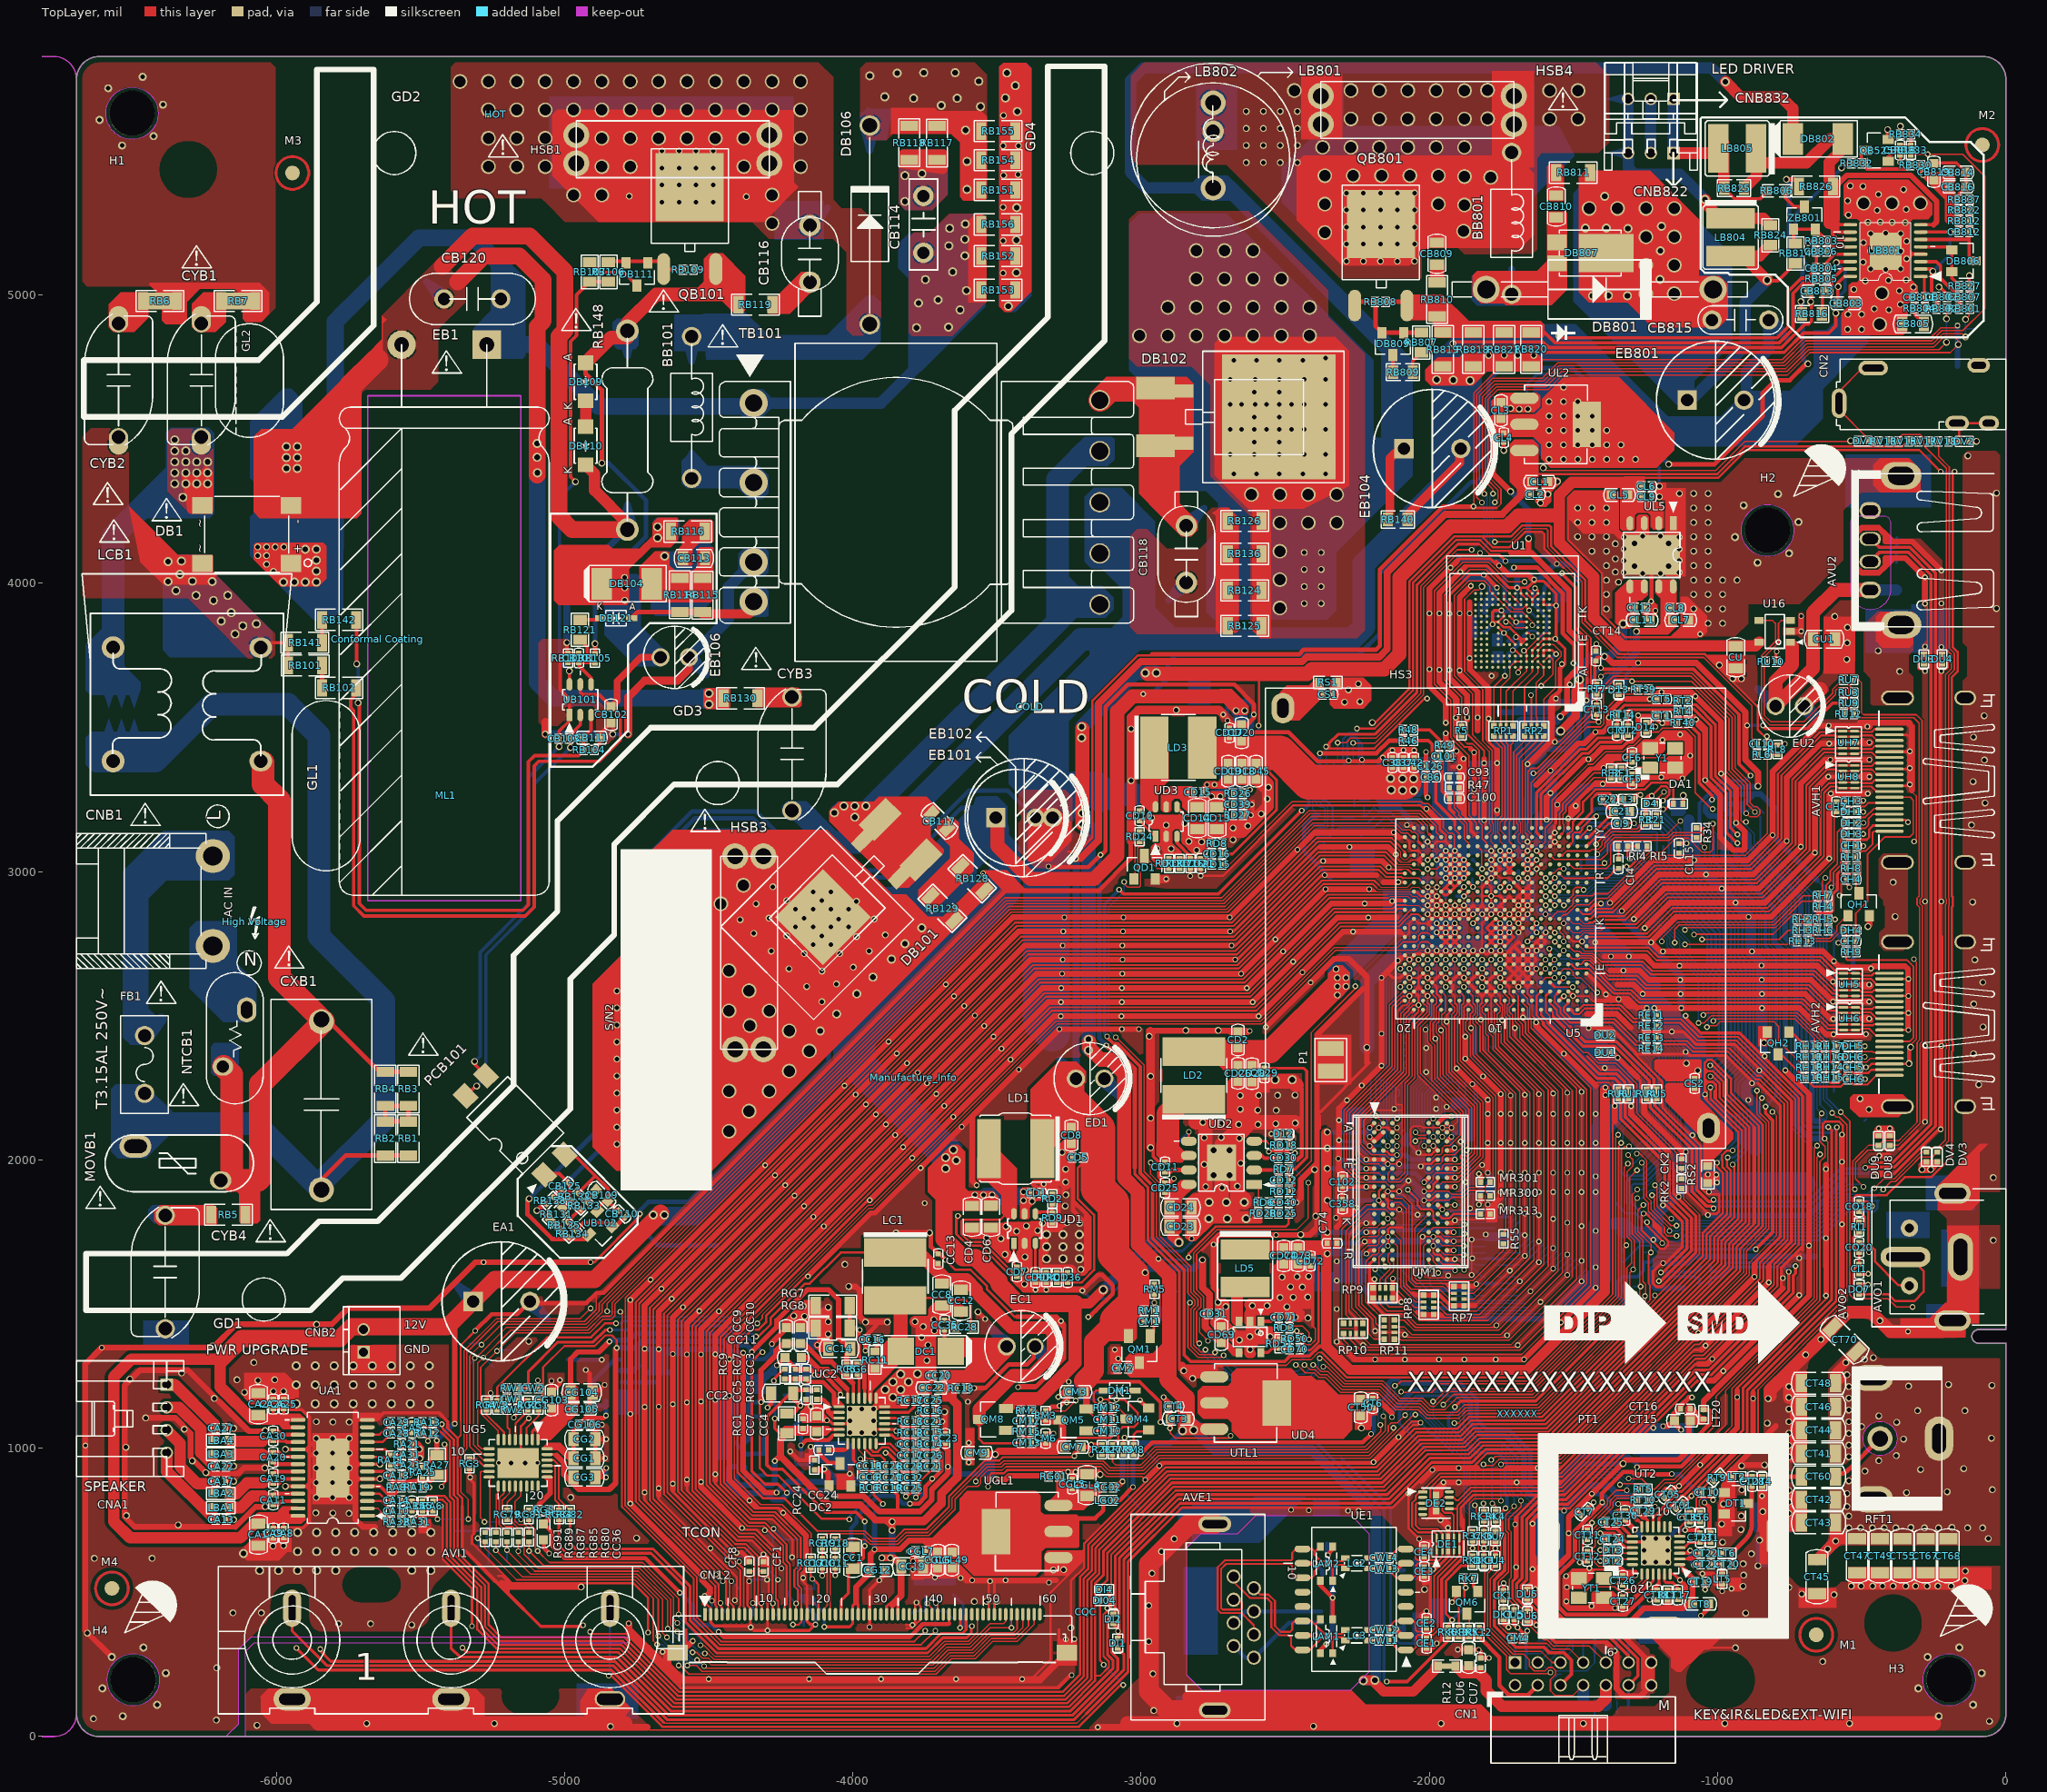
[diagram p0: TopLayer view]
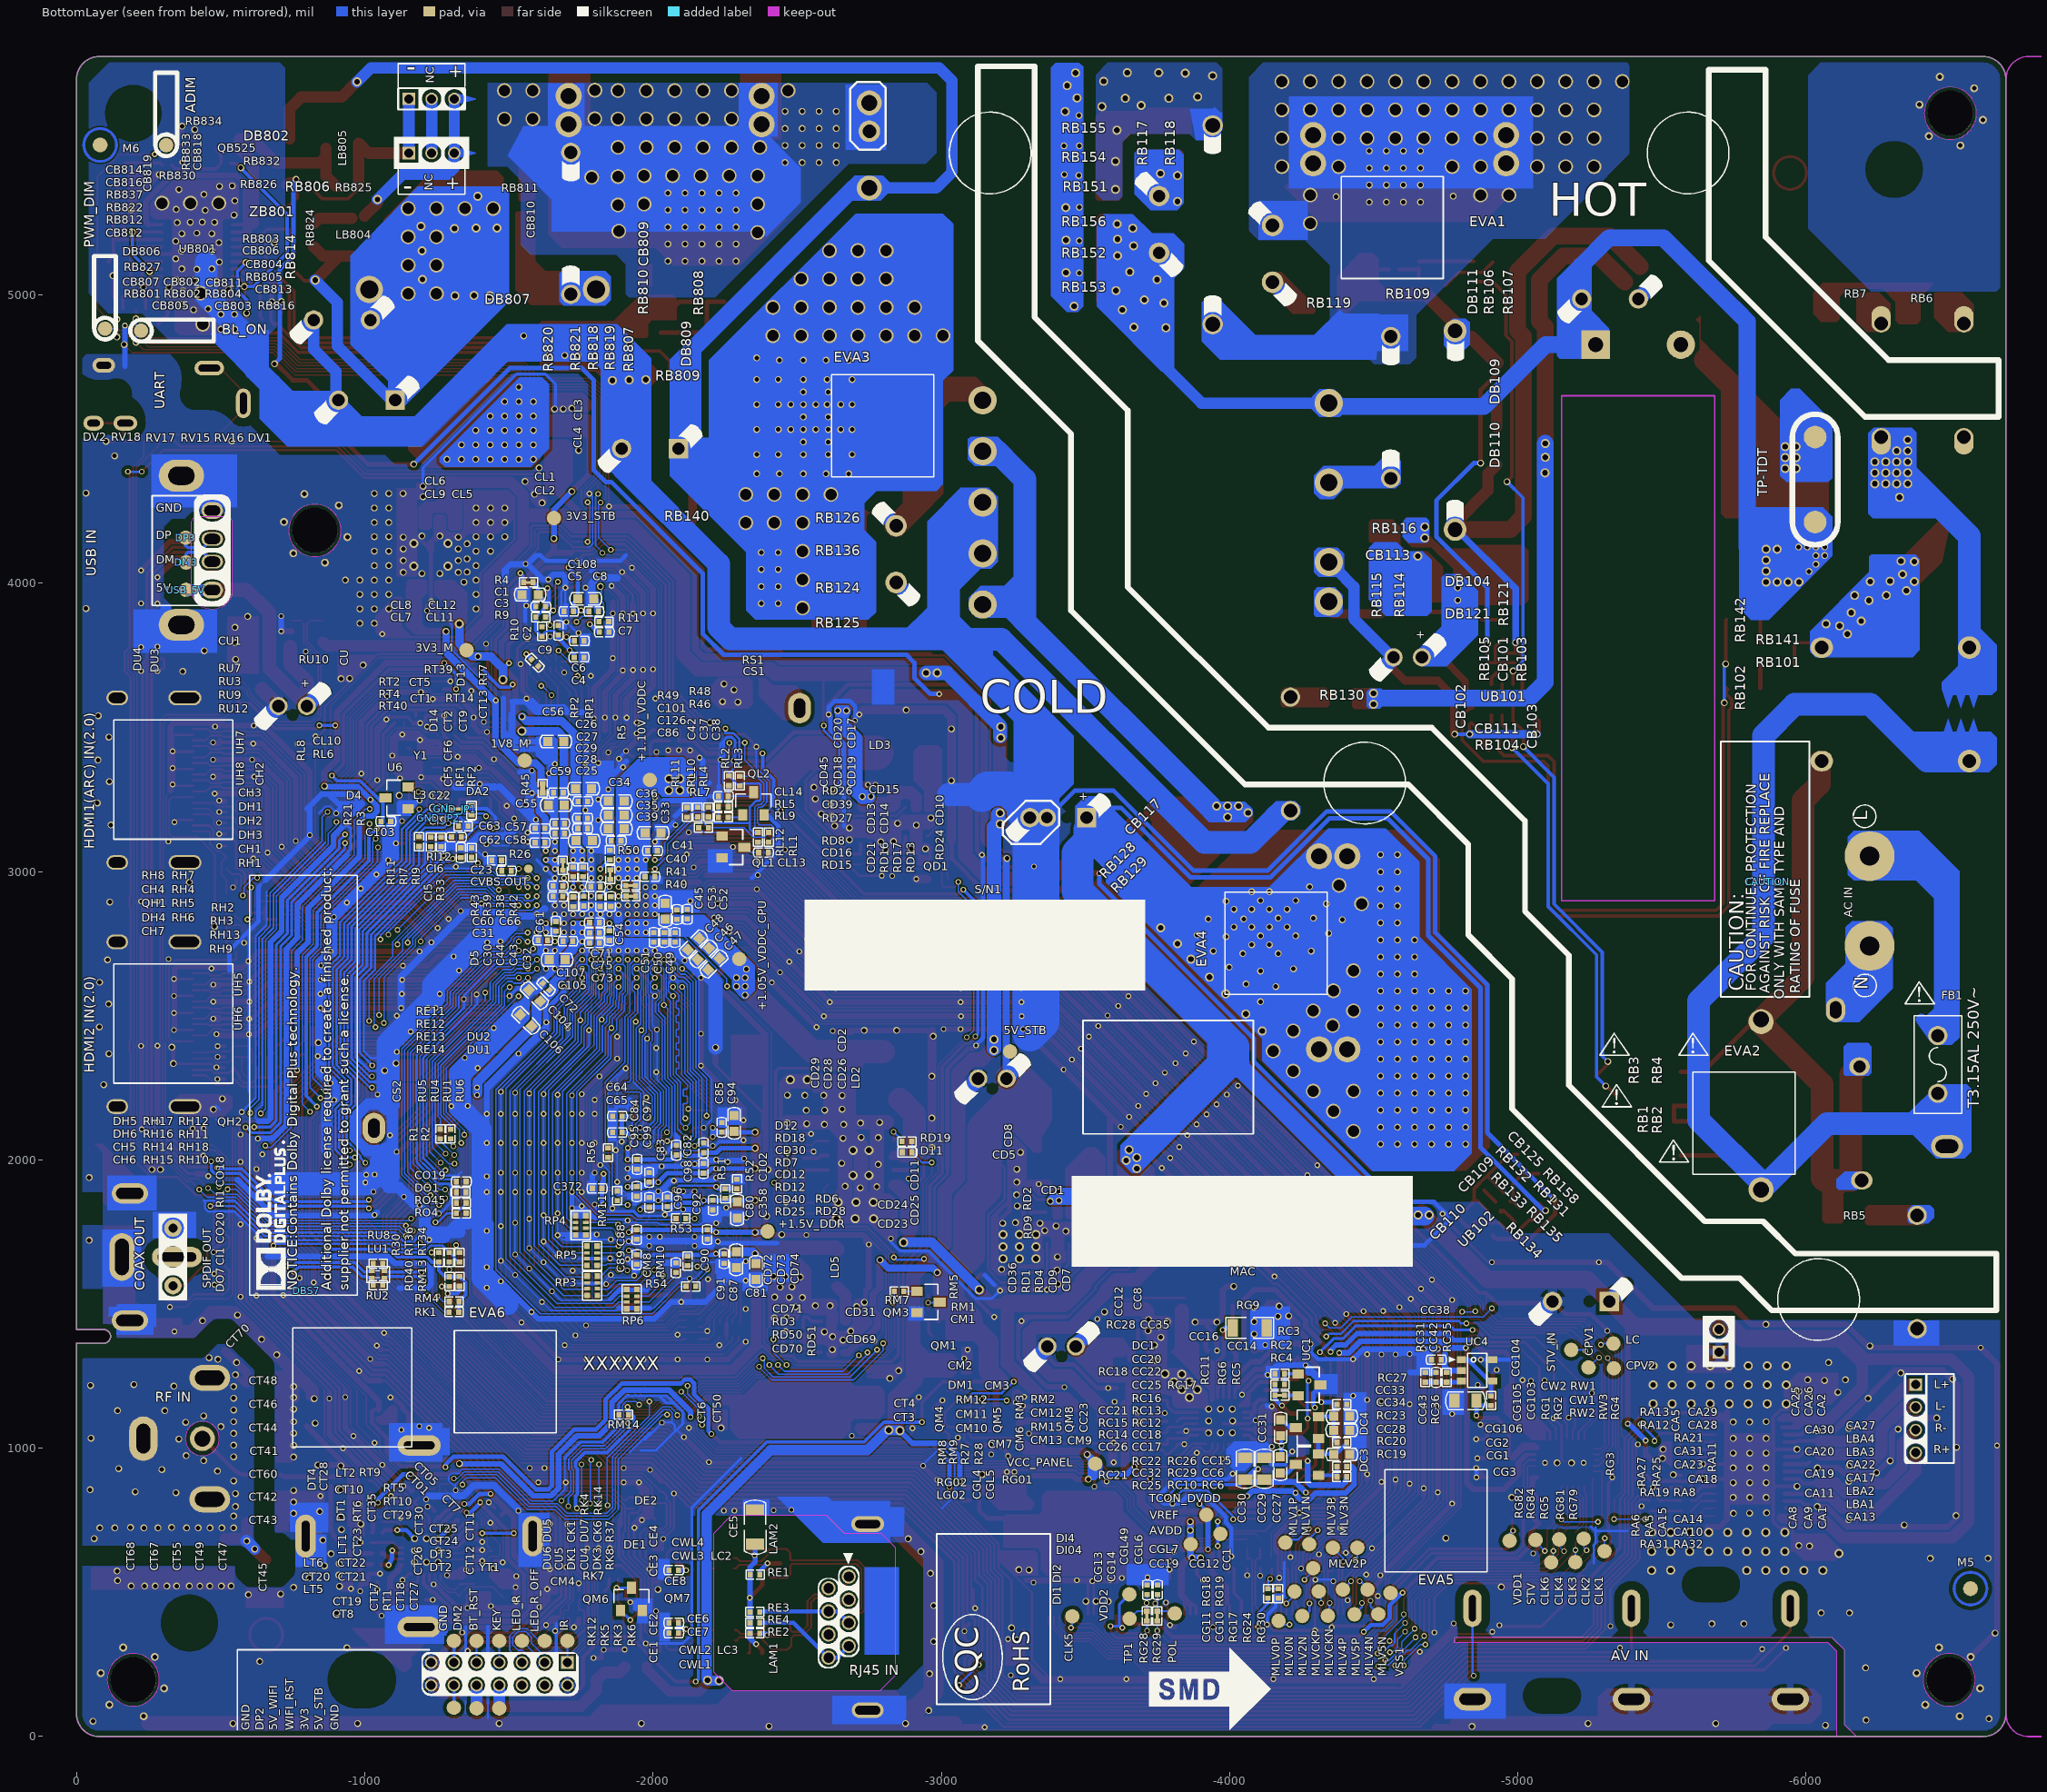
[diagram p1: BottomLayer view, seen from below]
# Altium PCB MISC84395.PcbDoc (part 1 of 26)
Units mil, origin at the board's own origin, x right, y up, seen from the top; angles counter-clockwise.
Board outline 6692.91 x 5826.77 mil, 2 copper layers (TopLayer, BottomLayer), stack 61.855 mil thick; 951 components, 565 nets, 4374 pads, 1804 vias.
Unrouted connection lines stored in the file: 1.

## Layer stack, top to bottom
TopLayer: signal copper 1.4
Dielectric: core 59.055, FR-4, Dk 4.8
BottomLayer: signal copper 1.4

## Board outline
-6692.91,78.74 -6692.91,5748.03 cw(c-6614.17,5748.03) -6614.17,5826.77 -78.74,5826.77 cw(c-78.74,5748.03) 0,5748.03 0,1411.42 -94.49,1411.42 ccw(c-94.49,1387.8) -118.11,1387.8 ccw(c-94.49,1387.8) -94.49,1364.17 0,1364.17 0,78.74 cw(c-78.74,78.74) -78.74,0 -6614.18,0 -6614.17,0 cw(c-6614.17,78.74)

## Design rules (kind name [scope] priority, off if disabled: settings)
Clearance ■KEEPOUT_18mil [(IsTrack Or IsArc) And (AsMM(Width) < 1) And IsKeepOut vs Not IsPad] p1: gap=18
Clearance ■HOT_7.2mm [InNetClass('HOT') vs InNetClass('All Nets') And (Not InNetClass('HOT'))] p2: gap=283.46
Clearance ■DFM_NPTH_10mil [(IsPadHoleValid And (PadIsPlated=false) Or IsPad And ((AsMM(PadXSize_AllLayers) < 1) or (AsMM(PadYSize_AllLayers) < 1 )) And IsKeepout) OR HasFootprintPad('ASSE*','0') vs Not IsPad] p3: gap=10
Clearance ■DFM_20mil [(IsTrack or IsArc or IsPad) And IsKeepOut vs IsTrack or IsArc or InPoly] p4: gap=20
Clearance ■C_RJ45_2mm [InNetClass('RJ45') vs Not InNetClass('RJ45') AND InNet('*')] p5: gap=78.74
Clearance ■PWR_A12_8mil [((InNetClass('PWR_A12_8mil') or InNet('*12V*') or InNet('*24V*') or InNet('*PVCC*') or InNet('*19V*') or InNet('*AMP*POWER*') or InNet('*AMP*VCC*') or InNet('*VGH*') or InNet('AVDD') or InNet('AVDD_SOURCE')) And Not InNetClass('A12_8mil_EXC')) and Not IsPad vs Not InPoly] p6: gap=8
Clearance ■PS_L2All_3.2mm [InNet('L-1') vs InNet('*')] p7: gap=125.98
Clearance ■PS_L2LN_1.5mm [InNet('L') Or InNet('L-2') Or InNet('L-3') Or InNet('L-4') Or InNet('L-5') Or InNet('L-6') vs InNet('L-N') And Not(InNet('L') Or InNet('L-2') Or InNet('L-3') Or InNet('L-4') Or InNet('L-5') Or InNet('L-6'))] p8: gap=59.06
Clearance ■PS_N2LN_1.5mm [InNet('N') OR InNet('N-1') OR InNet('N-2') OR InNet('N-3') OR InNet('N-4') OR InNet('N-5') OR InNet('N-6') vs InNet('L-N') And Not (InNet('N') OR InNet('N-1') OR InNet('N-2') OR InNet('N-3') OR InNet('N-4') OR InNet('N-5') OR InNet('N-6'))] p9: gap=59.06
Clearance ■PS_L2LN_3mm [InNet('L') Or InNet('L-2') Or InNet('L-3') Or InNet('L-4') Or InNet('L-5') Or InNet('L-6') vs InNet('*') And Not (InNet('L-N') Or InNet('L') Or InNet('L-2') Or InNet('L-3') Or InNet('L-4') Or InNet('L-5') Or InNet('L-6') Or OnLayer('KeepOutLayer'))] p10: gap=118.11
Clearance ■PS_N2LN_3mm [InNet('N') OR InNet('N-1') OR InNet('N-2') OR InNet('N-3') OR InNet('N-4') OR InNet('N-5') OR InNet('N-6') vs InNet('*') And Not (InNet('L-N') Or InNet('N') OR InNet('N-1') OR InNet('N-2') OR InNet('N-3') OR InNet('N-4') OR InNet('N-5') OR InNet('N-6') Or OnLayer('KeepOutLayer'))] p11: gap=118.11
Clearance ■SIP2GND_8mil [HasFootprint('SIP*') vs InPoly] p12: gap=8
Clearance ■C_BGA_0P65 [HasFootprint('BGA*0.65*') vs InPoly] p13: gap=5
Clearance ■C_BGA_0P8 [HasFootprint('BGA*0.8*') vs InPoly] p14: gap=5.5
Clearance ■Poly_4mil [InPolygonClass('Poly_4mil') vs Not InPoly] p15: gap=4
Clearance ■Poly_5mil [InPolygonClass('Poly_5mil') vs Not InPoly] p16: gap=5
Clearance ■Poly_6.2mil [InPolygonClass('Poly_6.2mil') vs Not InPoly] p17: gap=6.2
Clearance ■Poly_8mil [InPolygonClass('Poly_8mil') vs Not InPoly] p18: gap=8
Clearance ■C_RFGND_1.8mm [InNet('RFGND') vs Not (InNet('*RF*IN*') OR InNet('RF'))] p19: gap=70.87
Clearance ■ESD_10mil [HasFootprint('*IEC*') Or HasFootprint('*-F1*') Or HasFootprint('ANT-RF*')] p20: gap=10
Clearance ■ESD_20mil [HasFootprint('*SHIELD*')] p21: gap=20
Clearance ■GND_12mil [InNet('GND') vs InPoly] p22: gap=12
Clearance ■ESD_30mil [(HasFootprint('SCART*') OR HasFootprint('AV*') OR HasFootprint('DB15*') OR HasFootprint('PHONE*')) vs OnBottomLayer] p23: gap=30
Clearance ■ESD_NT_30mil [HasFootprint('SCART*') Or HasFootprint('PHONE-HD-12') Or HasFootprint('PHONE-HD-17') Or HasFootprint('PHONE-HD-10') Or HasFootprint('PHONE-HD-26') vs InNet('GND') And OnTopLayer] p24: gap=30
Clearance ■DFM_TH_5mil [HasFootprint('GND') or HasFootprint('TP*') or HasFootprint('MARK*') or HasFootprint('SPARK_GAP') or HasFootprint('USB-HD-3-2') or HasFootprint('PHONE-HS-20') and Not IsRegion vs OnBottomlayer And IsPad OR IsPadHoleValid] p25: gap=5
Clearance ■DFM_HS60_5mil [InPadClass('HS60') vs InPadClass('HS60') OR IsPadHoleValid and not InPadClass('VIA5')] p26: gap=5
Clearance ■DFM_BCR_4mm [IsPadHoleValid vs IsBoardCutoutRegion] p27: gap=157.48
Clearance ■DFM_TH_4mm [OnBottomlayer And IsSMTPin vs IsPadHoleValid and not InPadClass('VIA5')] p28: gap=157.48
Clearance ■DFM_HS60_4mm [InPadClass('HS60') vs IsPad and OnBottomlayer] p29: gap=157.48
Clearance ■VIA2VIA_6.2mil [(IsVia OR InPadClass('VIA5')) And Not (IsVia And (AsMM(HoleDiameter) = 0.1)) vs (IsVia OR InPadClass('VIA5')) And Not (IsVia And (AsMM(HoleDiameter) = 0.1))] p30: gap=6.2
Clearance ■VIA2VIA_10.2mil [(IsVia OR InPadClass('VIA5')) And Not (IsVia And (AsMM(HoleDiameter) = 0.1)) vs (IsVia OR InPadClass('VIA5')) And Not (IsVia And (AsMM(HoleDiameter) = 0.1))] p31: gap=10.2
Clearance ■VIA2PAD_BGA_5mil [HasFootprint('BGA*') and IsPad vs (IsVia OR InPadClass('VIA5')) And Not (IsVia And (AsMM(HoleDiameter) = 0.1))] p32: gap=4
Clearance ■VIA2PAD_6mil [IsVia And Not (IsVia And (AsMM(HoleDiameter) = 0.1)) vs ISPAD and Not HasFootprintPad('*','EPAD') and Not HasFootprintPad('*','257') and Not HasFootprintPad('TP','*') and Not HasFootprintPad('GND','JP*') and Not HasFootprintPad('LQFP216/0.4-2','217') and Not HasFootprintPad('QFP16*','17') and Not HasFootprintPad('QFN16*','17') and Not HasFootprintPad('QFN20*','21') and Not HasFootprintPad('QFN24*','25') and Not HasFootprintPad( 'QFN24*','29') and Not HasFootprintPad('QFN28*','29') and Not HasFootprintPad('QFN32*','33') and Not HasFootprintPad('QFN36*','37') and Not HasFootprintPad('QFN36*','0') and Not HasFootprintPad('QFN32*','0') and Not HasFootprintPad('QFN40*','41') and Not HasFootprintPad('QFN48*','49') and Not HasFootprintPad('LQFP48/0.5-2','49') and Not HasFootprintPad('*SSOP32*','33') and Not HasFootprintPad('SOP8*','9') and Not HasFootprintPad('WSON8/1.27*','9') and Not HasFootprintPad('DFN10/0.5-1*','11') and Not HasFootprintPad('SON16/0.4','9') and Not HasFootprintPad('MSOP10/0.5-1','11') and Not HasFootprintPad('QFN56/0.5','57') and Not HasFootprintPad('LGA31/0.5','3*') and Not InPadClass('VIA_HS60') and Not HasFootprintPad('TSSOP16/0.65-3','17') and Not HasFootprintPad('QFP128/0.5-2','129') and Not HasFootprintPad('QFP128/0.4-5','129') and Not HasFootprintPad('PQFP48*','49') and Not HasFootprintPad('QFP156/0.4-1','157') and Not HasFootprintPad('D2PAK3-TO-252','2') and Not HasFootprintPad('D2PAK3','2')] p33: gap=6
Clearance ■PAD2VIA5_6mil [IsPad And ((AsMM(PadXSize_AllLayers) < 2.5) or ((AsMM(PadYSize_AllLayers) < 2.5))) And Not InPadclass('HS60') vs InPadClass('VIA5')] p34: gap=6
Clearance "■12mil for Polygon" [InPoly] p35: gap=12
Clearance 8mil [All] p36 off: gap=8
Clearance 7mil [All] p37 off: gap=7
Clearance 6.2mil [All] p38 off: gap=6.2
Clearance 6mil [All] p39 off: gap=6
Clearance 5.8mil [All] p40 off: gap=5.8
Clearance 5mil [Not ((IsTrack Or IsArc) And (Layer = 'KeepOutLayer')) vs Not (IsPad or ((IsTrack Or IsArc) And (Layer = 'KeepOutLayer')))] p41 off: gap=5
Clearance 4.5mil [Not ((IsTrack Or IsArc) And (Layer = 'KeepOutLayer')) vs Not (IsPad or ((IsTrack Or IsArc) And (Layer = 'KeepOutLayer')))] p42 off: gap=4.5
Clearance 4mil [Not ((IsTrack Or IsArc) And (Layer = 'KeepOutLayer')) vs Not (IsPad or ((IsTrack Or IsArc) And (Layer = 'KeepOutLayer')))] p43 off: gap=4
Clearance "3.9mil for Minimum" [Not ((IsTrack Or IsArc) And (Layer = 'KeepOutLayer')) vs Not (IsPad or ((IsTrack Or IsArc) And (Layer = 'KeepOutLayer')))] p44: gap=3.9
ComponentClearance ■DFMC_1mm [Not (InComponentClass('Co-Layout') Or HasFootprint('GND')) And (HasFootprint('T/E*') Or HasFootprint('T/PQ*') Or HasFootprint('USB*') Or HasFootprint('HDMI*') Or HasFootprint('USB*') Or HasFootprint('DC-*') Or HasFootprint('AV*') Or HasFootprint('ANT*') Or HasFootprint('PHONE*') Or HasFootprint('CICARD*') Or HasFootprint('CARD*') Or HasFootprint('DVI*') Or HasFootprint('DB*') Or HasFootprint('DP*') Or HasFootprint('DISPLAYPORT*') Or HasFootprint('OPTICAL*') Or HasFootprint('SCART*') Or HasFootprint('RJ45*') Or HasFootprint('USB*') Or HasFootprint('T-*') Or HasFootprint('T/*') Or HasFootprint('200-*') Or HasFootprint('ZhiJia*') Or HasFootprint('Dianpian*') Or HasFootprint('TanPian*') Or HasFootprint('P(*')) vs Not (InComponentClass('Co-Layout') Or HasFootprint('GND'))] p1 off: gap=39.37 collisioncheckmode=3 verticalgap=39.37 showdistances=FALSE
ComponentClearance ■DFMC_0.5mm [Not (InComponentClass('Co-Layout') Or HasFootprint('SO-23') Or HasFootprint('DIODE-s0402') Or HasFootprint('GND')) And (HasFootprint('M-*') Or HasFootprint('BGA*') Or HasFootprint('QFP*') Or HasFootprint('QFN*') Or HasFootprint('*DFN*') Or HasFootprint('*SOP*') Or HasFootprint('LGA*') Or HasFootprint('SOIC*') Or HasFootprint('EC*') Or HasFootprint('AC-*') Or HasFootprint('DIODE*') Or HasFootprint('XTAL*') Or HasFootprint('SO-*') Or HasFootprint('L/LC*') Or HasFootprint('L(*') Or HasFootprint('WIFI*') Or HasFootprint('SATA*') Or HasFootprint('POGO*') Or HasFootprint('SOT-223') Or HasFootprint('TO-252') Or HasFootprint('TO-263') Or HasFootprint('KEY*') Or HasFootprint('SW*') Or HasFootprint('DIP*') Or HasFootprint('SIP*') Or HasFootprint('DIP*') Or HasFootprint('CON*') Or HasFootprint('FFC*') Or HasFootprint('FPC*') Or HasFootprint('GDT*') Or HasFootprint('R2512*') Or HasFootprint('R2725*') Or HasFootprint('L2012*') Or HasFootprint('L2520*')) vs Not (InComponentClass('Co-Layout') Or HasFootprint('SO-23') Or HasFootprint('DIODE-s0402') Or HasFootprint('GND'))] p2 off: gap=19.68 collisioncheckmode=3 verticalgap=19.68 showdistances=FALSE
ComponentClearance ■DFMC_0.4mm [Not (InComponentClass('Co-Layout') Or HasFootprint('GND')) And (HasFootprint('C0201*') Or HasFootprint('C0402*') Or HasFootprint('C0603*') Or HasFootprint('C0805*') Or HasFootprint('C1206*') Or HasFootprint('C1210*') Or HasFootprint('R0201*') Or HasFootprint('R0402*') Or HasFootprint('R0603*') Or HasFootprint('R0805*') Or HasFootprint('R*0402*') Or HasFootprint('L0201*') Or HasFootprint('L0402*') Or HasFootprint('L0603*') Or HasFootprint('L0805*') Or HasFootprint('L1206*') Or HasFootprint('DIODE-s0402')) vs Not (InComponentClass('Co-Layout') Or HasFootprint('GND')) And (HasFootprint('C0201*') Or HasFootprint('C0402*') Or HasFootprint('C0603*') Or HasFootprint('C0805*') Or HasFootprint('C1206*') Or HasFootprint('C1210*') Or HasFootprint('R0201*') Or HasFootprint('R0402*') Or HasFootprint('R0603*') Or HasFootprint('R0805*') Or HasFootprint('R*0402*') Or HasFootprint('L0201*') Or HasFootprint('L0402*') Or HasFootprint('L0603*') Or HasFootprint('L0805*') Or HasFootprint('L1206*') Or HasFootprint('DIODE-s0402'))] p3 off: gap=15.75 collisioncheckmode=3 verticalgap=15.75 showdistances=FALSE
ComponentClearance ■DFMC_0.36mm [Not (InComponentClass('Co-Layout') Or HasFootprint('GND')) And HasFootprint('R1206*') vs Not (InComponentClass('Co-Layout') Or HasFootprint('GND')) And HasFootprint('R1206*')] p4 off: gap=14.17 collisioncheckmode=3 verticalgap=14.17 showdistances=FALSE
ComponentClearance ■DFMC_0.25mm [Not (InComponentClass('Co-Layout') Or HasFootprint('GND')) vs Not (InComponentClass('Co-Layout') Or HasFootprint('GND'))] p5 off: gap=9.84 collisioncheckmode=3 verticalgap=9.84 showdistances=FALSE
DiffPairsRouting ■DiffPair_USB_DiffPairsRouting [InDifferentialPairClass('USB')] p1: maxlimit=5 minlimit=4 mostfreqgap=5 maxuncoupledlength=200
DiffPairsRouting ■DiffPair_LVDS_DiffPairsRouting [InDifferentialPairClass('LVDS')] p2: maxlimit=5 minlimit=4 mostfreqgap=5 maxuncoupledlength=500
DiffPairsRouting ■DiffPair_HDMI_DiffPairsRouting [InDifferentialPairClass('HDMI')] p3: maxlimit=5 minlimit=4 mostfreqgap=5 maxuncoupledlength=200
DiffPairsRouting [All] p4: maxlimit=10 minlimit=10 mostfreqgap=10 maxuncoupledlength=500
FabricationTestPointUsage TestPointUsage [All] p1: valid=0 allowmultiple=FALSE
FabricationTestpoint Testpoint [All] p1: side=3 testpointundercomponent=TRUE minsize=40 maxsize=100 preferedsize=60 minholesize=20 maxholesize=40 preferedholesize=32 testpointgrid=1 allowsidetop=TRUE allowsidebottom=TRUE usegrid=TRUE gridtolerance=0.01
HoleSize HoleSize_VIA [ISVIA] p1 off: absolutevalues=TRUE maxlimit=23.62 minlimit=7.87 maxpercent=80.000 minpercent=20.000
HoleToHoleClearance Hole2Hole [All] p1 off: gap=18 allowstackedmicrovias=FALSE
MatchedLengths DiffPair_USB_MatchedLengths [InDifferentialPairClass('USB')] p1: tolerance=100 checknetsindiffpair=TRUE checkdiffpairvsdiffpair=FALSE checkothers=FALSE
MatchedLengths DiffPair_LVDS_MatchedLengths [InDifferentialPairClass('LVDS')] p2: tolerance=100 checknetsindiffpair=TRUE checkdiffpairvsdiffpair=FALSE checkothers=FALSE
MatchedLengths DiffPair_HDMI_MatchedLengths [InDifferentialPairClass('HDMI')] p3: tolerance=100 checknetsindiffpair=TRUE checkdiffpairvsdiffpair=FALSE checkothers=FALSE
MinimumAnnularRing [All] p1: minimumring=3.94
MinimumSolderMaskSliver ■MiniSolderMaskSliver [All] p1 off: minsoldermaskwidth=3.87
NetAntennae [Not (HasFootprint('ANT-7') or HasFootprint('ANT-BLUECORE'))] p1: netantennaetolerance=40
PermittedLayers [All] p1: toplayerpermitted=TRUE bottomlayerpermitted=TRUE
PlaneClearance ■Plane_ESD_30mil [(HasFootprint('SCART*') OR HasFootprint('AV*') OR HasFootprint('DB15*') OR HasFootprint('PHONE*'))] p1: clearance=30
PlaneClearance ■Plane_All_9mil [All] p2: clearance=9
PlaneConnect ■PlaneOverAll [IsVia or InPadClass('VIA5') Or HasFootprint('ASSE*') OR InPadclass('HS60')] p1: planeconnectstyle=Direct reliefexpansion=20 reliefentries=4 reliefconductorwidth=10 reliefairgap=10
PlaneConnect ■PlaneConnect [All] p2: planeconnectstyle=Relief reliefexpansion=12 reliefentries=4 reliefconductorwidth=30 reliefairgap=12
PolygonConnect ■PourOverAll [IsVia Or InPadclass('HS60') Or InPadClass('VIA5') Or HasFootprint('ASSE*') Or HasFootprint('DIODE-S0402') Or HasFootprint('RCL0524P') Or HasFootprint('SOT-89') OR HasFootprint('SOT-223') OR HasFootprint('TO-252') OR HasFootprint('TO-263') OR HasFootprint('DIODE') OR HasFootprint('SW-HS-2') OR HasFootprint('HDMI*') OR HasFootprint('SO-8B') OR HasFootprint('GND') OR HasFootprint('PHONE*') OR HasFootprint('DIP18/2.54-2') OR HasFootprint('DIP18/2.54-1') OR HasFootprint('UFL-R-SMT-1') OR HasFootprint('WIFI') OR HasFootprint('UM02BS') OR HasFootprint('*SCART*') OR HasFootprint('TSOT23-8/0.65') OR HasFootprint('*SOT-23-*') OR HasFootprint('SOP23-5-1') OR HasFootprint('SOP6/0.95') OR HasFootprint('M-WIFI-2-M603USA1') OR HasFootprint('M-MT7632U') OR HasFootprint('SOP8/1.27') OR HasFootprint('SOP8/1.27-3') vs IsPolygon] p1: connectstyle=Direct reliefconductorwidth=10 reliefentries=4 polygonreliefangle="90 Angle"
PolygonConnect ■BGA_0P65 [HasFootprint('BGA*0.65*') vs IsPoly] p2: connectstyle=Relief reliefconductorwidth=8 reliefentries=4 polygonreliefangle="45 Angle"
PolygonConnect ■BGA_0P8 [HasFootprint('BGA*0.8*') vs IsPoly] p3: connectstyle=Relief reliefconductorwidth=9 reliefentries=4 polygonreliefangle="45 Angle"
PolygonConnect ■Polygon_RFGND [InNet('RFGND')] p4: connectstyle=Direct reliefconductorwidth=10 reliefentries=4 polygonreliefangle="90 Angle"
PolygonConnect ■ESD_SCART [HasFootprint('SCART*') vs IsPolygon And onBottomlayer] p5: connectstyle=Direct reliefconductorwidth=30 reliefentries=4 polygonreliefangle="90 Angle"
PolygonConnect ■C2Polygon_35mil [HasFootprint('EC*') vs IsPolygon] p6: connectstyle=Relief reliefconductorwidth=35 reliefentries=4 polygonreliefangle="90 Angle"
PolygonConnect ■C2Polygon_30mil [(HasFootprint('*0805*') OR HasFootprint('*1206*')) vs IsPolygon] p7: connectstyle=Relief reliefconductorwidth=30 reliefentries=4 polygonreliefangle="90 Angle"
PolygonConnect ■C2Polygon_25mil [HasFootprint('*0603*') Or IsThruPin vs IsPolygon] p8: connectstyle=Relief reliefconductorwidth=25 reliefentries=4 polygonreliefangle="90 Angle"
PolygonConnect ■C2Polygon_12mil [IsSMTPin vs IsPolygon] p9: connectstyle=Relief reliefconductorwidth=12 reliefentries=4 polygonreliefangle="90 Angle"
RoomDefinition MS348T [InComponentClass('MS348T')] p1: confinementstyle=ConfineIn formatcopy=TRUE lockcomponents=FALSE outline -2111.65,3200.74 -2131.65,3180.74 -2131.65,2494.74 -2111.65,2474.74 -1428.15,2474.74 -1404.65,2498.24 -1404.65,3181.24 -1424.15,3200.74
RoutingVias 0.6_0.4 [All] p1 off: holewidth=15.75 width=23.62 viastyle="Through Hole" minholewidth=15.75 minwidth=23.62 maxholewidth=15.75 maxwidth=23.62
RoutingVias 0.8_0.5 [All] p2 off: holewidth=19.68 width=31.5 viastyle="Through Hole" minholewidth=19.68 minwidth=31.5 maxholewidth=19.68 maxwidth=31.5
RoutingVias 0.5_0.3 [All] p3: holewidth=11.81 width=19.68 viastyle="Through Hole" minholewidth=11.81 minwidth=19.68 maxholewidth=11.81 maxwidth=19.68
RoutingVias 0.45_0.25 [All] p4 off: holewidth=9.84 width=17.72 viastyle="Through Hole" minholewidth=9.84 minwidth=17.72 maxholewidth=9.84 maxwidth=17.72
RoutingVias 0.4_0.2 [All] p5 off: holewidth=7.87 width=15.75 viastyle="Through Hole" minholewidth=7.87 minwidth=15.75 maxholewidth=7.87 maxwidth=15.75
RoutingVias 0.25_0.1 [All] p6 off: holewidth=3.94 width=9.84 viastyle="Through Hole" minholewidth=3.94 minwidth=9.84 maxholewidth=3.94 maxwidth=9.84
SMDNeckDown ■SMDNeckDown_Chip [HasFootprint('FFC*') or HasFootprint('QFP*') or HasFootprint('QFN*') or HasFootprint('HDMI*') or HasFootprint('BGA*')] p1: percent=100.000
SMDToCorner [All] p1 off: distance=40000
ShortCircuit ■ShortCircuit_ViaOnEpad [HasFootprintPad( '*','EPAD') vs IsVia AND InNet('*')] p1: allowed=TRUE
ShortCircuit ■ShortCircuit_JP [HasFootprintPad( 'GND','JP_1K') vs HasFootprintPad( 'GND','JP_2K')] p2: allowed=TRUE
ShortCircuit ■ShortCircuit_0402 [HasFootprintPad('R0402SC','1') OR HasFootprintPad('R0402SC','2') vs HasFootprintPad('R0402SC','3')] p3: allowed=TRUE
ShortCircuit ■ShortCircuit_0603 [HasFootprintPad('R0603SC','1') OR HasFootprintPad('R0603SC','2') vs HasFootprintPad('R0603SC','3')] p4: allowed=TRUE
ShortCircuit ■ShortCircuit_0805 [HasFootprintPad('R0805SC','1') OR HasFootprintPad('R0805SC','2') vs HasFootprintPad('R0805SC','3')] p5: allowed=TRUE
ShortCircuit ■ShortCircuit_1206 [HasFootprintPad('R1206SC','1') OR HasFootprintPad('R1206SC','2') vs HasFootprintPad('R1206SC','3')] p6: allowed=TRUE
ShortCircuit ■ShortCircuit [InNet('*')] p7: allowed=FALSE
SilkToSilkClearance ■Silk2Silk [All] p1: silktosilkclearance=5
SilkscreenOverComponentPads ■SilkOverPads [IsText] p1: minsilkscreentomaskgap=0.1
SolderMaskExpansion ■SolderMask_VIA [IsVia] p1: expansion=5.1
SolderMaskExpansion ■SolderMask_All [All] p2: expansion=2
UnRoutedNet ■UnRoutedNet [All] p1:
ViasUnderSMD [All] p1: allowed=FALSE
Width ■Width_2.5mm [InFromToClass('Width_2.5mm')] p1: maxlimit=98.43 minlimit=98.43 preferedwidth=98.43
Width ■Width_1.5mm [InFromToClass('Width_1.5mm')] p2: maxlimit=59.06 minlimit=59.06 preferedwidth=59.06
Width ■DiffPair_USB_Width [InDifferentialPairClass('USB')] p3: maxlimit=11 minlimit=4 preferedwidth=11
Width ■DiffPair_LVDS_Width [InDifferentialPairClass('LVDS')] p4: maxlimit=7 minlimit=4 preferedwidth=7
Width ■DiffPair_HDMI_Width [InDifferentialPairClass('HDMI')] p5: maxlimit=7 minlimit=4 preferedwidth=7
Width [All] p6: maxlimit=500 minlimit=3 preferedwidth=8
14 further rules are at their usual default settings.

## Classes and differential pairs
net class POWER: 12V 12V_OVP ADIM BL_ON BRO D_QB101 D_QB801 GND L L-1 L-2 L-N LED+ LED- LED_CS LED_FB LED_GATE LED_OVP N N-1 N-2 NetBB101_2 NetBB801_2 NetCB101_1 NetCB102_1 NetCB103_1 NetCB109_1 NetCB109_2 NetCB110_2 NetCB113_1 NetCB113_2 NetCB114_1 NetCB116_1 NetCB117_1 NetCB117_2 NetCB118_1 NetCB118_2 NetCB125_1 NetCB125_2 NetCB802_2 NetCB804_2 NetCB805_2 NetCB807_1 NetCB809_1 NetCB810_1 NetCB811_1 NetCB812_2 NetCB813_2 NetCB814_1 NetCB815_1 NetCB818_2 NetCNB822_2 NetCYB3_1 NetCYB4_1 NetDB106_K NetDB109_A NetDB109_K NetDB111_1 NetDB111_2 NetDB121_K NetDB801_K NetDB806_1 NetDB809_1 NetDB809_2 NetHSB1_1 NetHSB1_3 NetHSB3_1 NetHSB3_3 NetHSB4_1 NetHSB4_3 NetQB525_B NetQB525_C NetRB101_2 NetRB106_1 NetRB141_1 NetRB151_2 NetRB806_2 PWM_DIM SGND UB801-VCC VBL VBRIDGE
net class HOT: 12V_OVP BRO D_QB101 L L-1 L-2 L-N N N-1 N-2 NetBB101_2 NetCB101_1 NetCB102_1 NetCB103_1 NetCB113_1 NetCB113_2 NetCB114_1 NetCB116_1 NetCB116_2 NetCYB3_1 NetCYB4_1 NetDB106_K NetDB109_A NetDB109_K NetDB111_1 NetDB111_2 NetDB121_K NetRB101_2 NetRB106_1 NetRB141_1 NetRB151_2 SGND VBRIDGE
component class TV#13_LevelShif: AVDD CC36 CF1 CF8 CG1 CG2 CG3 CG4 CG5 CG6 CG7 CG8 CG9 CG10 CG11 CG12 CG13 CG14 CG42 CG60 CG61 CG62 CG63 CG103 CG104 CG105 CG106 CLK1 CLK2 CLK3 CLK4 CLK5 CLK6 CN12 CPV1 CPV2 CW1 CW2 LC MLV0N MLV0P MLV1N MLV1P MLV2N MLV2P MLV3N MLV3P MLV4N MLV4P MLV5N MLV5P MLVCKN MLVCKP POL Q1 RG1 RG2 RG3 RG4 RG5 RG10 RG11 RG12 RG13 RG14 RG15 RG16 RG18 RG19 RG28 RG29 RG79 RG80 RG81 RG82 RG84 RG85 RG87 RG89 RG91 RW1 RW2 RW3 STV STV_IN TCON_DVDD TP1 UG1 UG5 VDD1 VDD2 VREF VSS1
component class TV#12_TCON: CC1 CC2 CC3 CC4 CC5 CC6 CC7 CC8 CC9 CC10 CC11 CC12 CC13 CC14 CC15 CC16 CC17 CC18 CC19 CC20 CC21 CC22 CC23 CC24 CC25 CC26 CC27 CC28 CC29 CC30 CC31 CC32 CC33 CC34 CC35 CC38 CC42 CC43 CGL4 CGL5 CGL6 CGL7 CGL49 CM10 CM11 DC1 DC2 DC3 DC4 DM1 EC1 LC1 LG02 RC1 RC2 RC3 RC4 RC5 RC6 RC7 RC8 RC9 RC10 RC11 RC12 RC13 RC14 RC15 RC16 RC17 RC18 RC19 RC20 RC21 RC22 RC23 RC24 RC25 RC26 RC27 RC28 RC29 RC31 RC35 RC36 RG01 RG02 RG6 RG7 RG8 RG9 RG17 RG24 RG30 RM12 UC1 UC2 UC4 UGL1
component class TV#11_Tuner: CT1 CT01 CT2 CT3 CT4 CT05 CT5 CT6 CT7 CT8 CT9 CT10 CT11 CT12 CT13 CT14 CT15 CT16 CT17 CT18 CT19 CT20 CT21 CT22 CT23 CT24 CT25 CT26 CT27 CT28 CT29 CT30 CT35 CT41 CT42 CT43 CT44 CT45 CT46 CT47 CT48 CT49 CT50 CT55 CT60 CT67 CT68 CT70 DT1 DT2 DT3 DT4 LT1 LT2 LT3 LT4 LT5 LT6 LT20 PT1 RFT1 RT1 RT2 RT4 RT5 RT6 RT7 RT9 RT10 RT14 UT2 UTL1 YT1
component class TV#10_AMP: CA1 CA2 CA5 CA8 CA9 CA10 CA11 CA13 CA14 CA15 CA17 CA18 CA19 CA20 CA22 CA23 CA25 CA26 CA27 CA28 CA29 CA30 CA31 CNA1 DA1 DA2 EA1 GND_JP1 GND_JP2 LBA1 LBA2 LBA3 LBA4 RA5 RA6 RA8 RA11 RA12 RA13 RA19 RA21 RA25 RA27 RA31 RA32 UA1
component class TV#09_KEY&IR: 5V_WIFI BT_RST CK1 CK2 CK6 CM4 CN1 CU4 CU5 CU6 CU7 DK1 DK3 DM2 DP2 DU5 DU6 DU7 IR KEY LED_R LED_R_OFF LU1 QM6 QM7 R12 RK1 RK2 RK3 RK4 RK5 RK6 RK7 RK8 RK12 RK14 RM13 RM14 RU1 RU2 RU6 RU8 WIFI_RST
component class TV#08_USB_Network: AVE1 AVU2 CE1 CE2 CE3 CE4 CE5 CE6 CE7 CE8 CU CU1 CWL1 CWL2 CWL3 CWL4 DE1 DE2 DM3 DP3 DU1 DU2 DU3 DU4 DU8 DU9 EU2 LAM1 LAM2 LC2 LC3 RE1 RE2 RE3 RE4 RE11 RE12 RE13 RE14 RU2 RU3 RU4 RU5 RU7 RU9 RU10 RU12 U16 UE1 USB_5V
component class TV#07_HDMI: AVH1 AVH2 CH1 CH2 CH3 CH4 CH5 CH6 CH7 DH1 DH2 DH3 DH4 DH5 DH6 QH1 QH2 RH1 RH2 RH3 RH4 RH5 RH6 RH7 RH8 RH9 RH10 RH11 RH12 RH13 RH14 RH15 RH16 RH17 RH18 UH5 UH6 UH7 UH8
component class TV#06_COXA&AV: AVI1 AVO1 AVO2 CI1 CI4 CI5 CI6 CI9 CO18 CO19 CO20 DI1 DI2 DI4 DI04 DO1 DO7 RI1 RI4 RI5 RI7 RI9 RI11 RI12 RO4 RO45
component class TV#05_EMMC: C1 C2 C3 C4 C5 C6 C7 C8 C9 C108 R4 R5 R9 R10 R11 RP1 RP2 U1
component class TV#04_MSD6A348_DRAM: C80 C81 C82 C83 C84 C85 C86 C87 C88 C89 C90 C91 C92 C93 C94 C95 C96 C97 C98 C99 C100 C101 C102 C126 C358 C372 CM8 MR300 MR301 MR313 R46 R47 R48 R49 R50 R51 R52 R53 R54 R55 R56 RM10 RM11 RP3 RP4 RP5 RP6 RP7 RP8 RP9 RP10 RP11 U5 UM1
component class TV#03_MSD6A348_Power: C25 C26 C27 C28 C29 C30 C31 C32 C33 C34 C35 C36 C37 C38 C39 C40 C41 C42 C43 C44 C45 C46 C47 C48 C49 C50 C51 C52 C53 C54 C55 C56 C57 C58 C59 C60 C61 C62 C63 C64 C65 C66 C71 C72 C73 C74 C75 C104 C105 C106 C107 D5 R38 R39 R40 R41 R42 R43 R45
component class TV#02_MSD6A348_SYS: C21 C22 C23 C103 CF5 CF6 CN2 "CVBS OUT" D4 D11 D12 D13 D14 DV1 DV2 DV3 DV4 L3 R1 R2 R3 R21 R26 R27 R28 R30 R33 R34 R37 RF1 RF2 RT34 RT36 RT39 RT40 RV15 RV16 RV17 RV18 RXE4N U6 VGPIN1 Y1
component class TV#01_SYSTEM_POWER: 1V8_M 3V3_M 3V3_STB 5V_STB +1.5V_DDR +1.05V_VDDC_CPU +1.10V_VDDC CD1 CD2 CD4 CD5 CD6 CD7 CD8 CD9 CD10 CD11 CD12 CD13 CD14 CD15 CD16 CD17 CD18 CD19 CD20 CD21 CD23 CD24 CD25 CD26 CD28 CD29 CD30 CD31 CD36 CD39 CD40 CD45 CD69 CD70 CD71 CD72 CD73 CD74 CL1 CL2 CL3 CL4 CL5 CL6 CL7 CL8 CL9 CL10 CL11 CL12 CL13 CL14 CL15 CM1 CM2 CM3 CM6 CM7 CM9 CM10 CM11 CM12 CM13 DM1 ED1 LD1 LD2 LD3 LD5 QD1 QL1 QL2 QM1 QM3 QM4 QM5 QM8 RD1 RD2 RD3 RD4 RD6 RD7 RD8 RD9 RD12 RD13 RD15 RD16 RD17 RD18 RD19 RD24 RD25 RD26 RD27 RD28 RD40 RD50 RD51 RL1 RL2 RL3 RL4 RL5 RL6 RL7 RL8 RL9 RL10 RL11 RL12 RM1 RM2 RM3 RM4 RM5 RM7 RM8 RM9 RM12 RM15 UD1 UD2 UD3 UD4 UL2 UL5 VCC_PANEL
component class SCH_info: CS1 CS2 DBS7 HS3 P1 RS1 RS2 XXXXXX XXXXXXXXXXXXXXXX 用于U5上